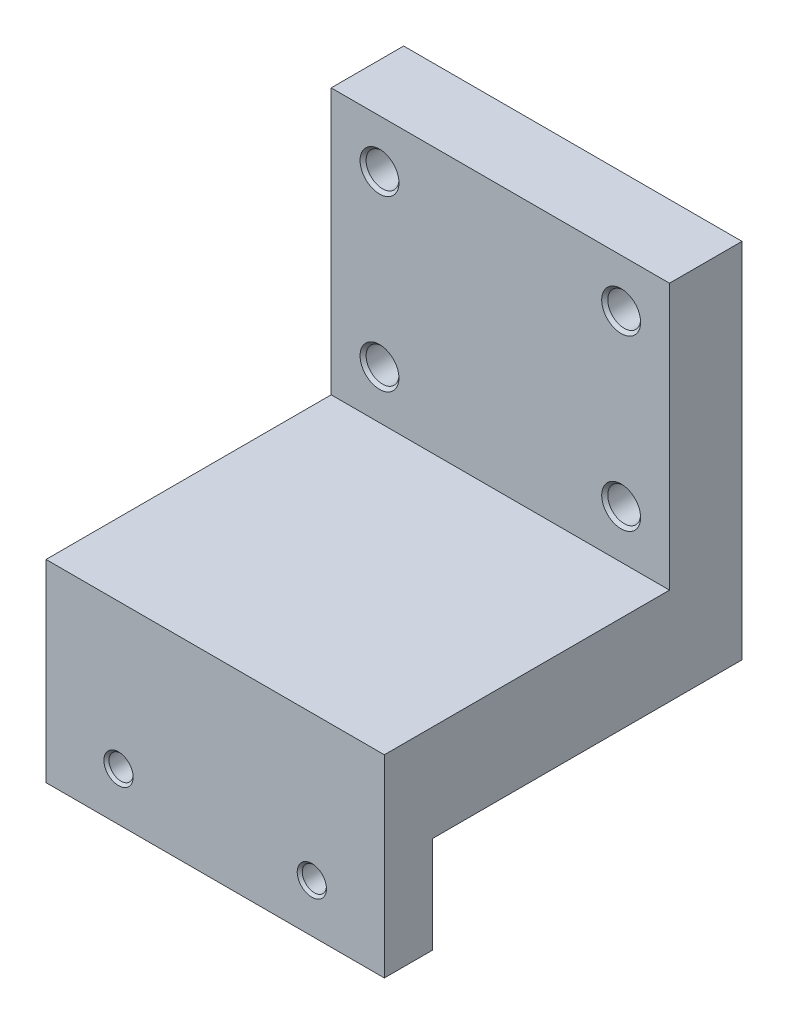
SolidWorks part; units mm, degrees
ref_plane "前视基准面" through (0, 0, 0) normal (0, 0, 1) x (1, 0, 0)
ref_plane "上视基准面" through (0, 0, 0) normal (0, 1, 0) x (1, 0, 0)
ref_plane "右视基准面" through (0, 0, 0) normal (1, 0, 0) x (0, 0, -1)
sketch "草图1" plane through (0, 0, 0) normal (0, 0, 1) x (1, 0, 0)
  line L0 (0, 0) -> (0, 45) construction
  line L1 (75, 35) -> (-75, 35) construction
  line L2 (-35, 55) -> (35, 55)
  line L3 (-35, 55) -> (-35, 35)
  line L4 (-35, 35) -> (35, 35)
  line L5 (35, 55) -> (35, 35)
  line L6 (-35, 55) -> (35, 35) construction
  line L7 (-35, 35) -> (35, 55) construction
  dimension "D1" = 20
  dimension "D2" = 70
extrude "凸台-拉伸1" add sketch "草图1" against normal blind 64 and the other way blind 10
sketch "草图2" plane through (0, 35, 0) normal (0, -1, 0) x (1, 0, 0)
  line L0 (35, 10) -> (35, -64) construction
  line L1 (-35, 10) -> (35, 10)
  line L2 (-35, 10) -> (-35, 0)
  line L3 (-35, 0) -> (35, 0)
  line L4 (35, 10) -> (35, 0)
  line L5 (-75, 0) -> (75, 0) construction
extrude "凸台-拉伸2" add sketch "草图2" along normal blind 20
sketch "草图3" plane through (0, 55, 0) normal (0, 1, 0) x (1, 0, 0)
  line L0 (-35, -10) -> (-35, 64) construction
  line L1 (35, 64) -> (-35, 64)
  line L2 (35, 64) -> (35, 49)
  line L3 (35, 49) -> (-35, 49)
  line L4 (-35, 64) -> (-35, 49)
  dimension "D1" = 15
extrude "凸台-拉伸3" add sketch "草图3" along normal blind 55
sketch "草图4" plane through (0, 0, -49) normal (0, 0, 1) x (1, 0, 0)
  line L8 (-25, 65) -> (25, 65)
  line L9 (25, 65) -> (25, 100)
  line L10 (25, 100) -> (-25, 100)
  line L11 (-25, 100) -> (-25, 65)
  line L12 (-25, 65) -> (25, 65)
  line L13 (25, 65) -> (25, 100)
  line L14 (25, 100) -> (-25, 100)
  line L15 (-25, 100) -> (-25, 65)
  dimension "D1" = 10
hole_wizard "M8 螺纹孔1" positions "草图7" profile "草图6" tap size "M8" standard "GB"
sketch "草图7" plane through (0, 0, -49) normal (0, 0, 1) x (1, 0, 0)
  point P0 (25, 100)
  point P3 (25, 65)
  point P6 (-25, 65)
  point P9 (-25, 100)
sketch "草图6" plane through (25, 100, -49) normal (1, 0, 0) x (0, -1, 0)
  line L0 (0, 0) -> (0, 19.75)
  line L1 (0, 19.75) -> (3.4, 17.7071)
  line L2 (3.4, 17.7071) -> (3.4, 0.625)
  line L3 (3.4, 0.625) -> (4.025, 0)
  line L5 (4.025, 0) -> (0, 0)
  line L6 (-3.4, 0.625) -> (-4.025, 0) construction
  line L10 (0, 19.75) -> (-3.4, 17.7071) construction
  line L11 (0, -6.35) -> (0, 107.95) construction
  dimension "螺纹孔钻头直径" = 6.8
  dimension "螺纹孔钻头深度" = 19.75
  dimension "近端锥形沉头孔直径" = 8.05
  dimension "近端锥形沉头孔角度" = 90
  dimension "导头角度" = 118
cosmetic thread "孔螺蚊线1" parameters "D1"=16, "D2"=8
cosmetic thread "孔螺蚊线2" parameters "D1"=16, "D2"=8
cosmetic thread "孔螺蚊线3" parameters "D1"=16, "D2"=8
cosmetic thread "孔螺蚊线4" parameters "D1"=16, "D2"=8
sketch "草图8" plane through (0, 0, 10) normal (0, 0, 1) x (1, 0, 0)
  line L0 (0, 0) -> (0, 25) construction
  line L1 (20, 25) -> (-20, 25)
  dimension "D1" = 20
  dimension "D2" = 25
hole_wizard "M6 螺纹孔1" positions "草图9" profile "草图10" tap size "M6" standard "GB"
sketch "草图9" plane through (0, 0, 10) normal (0, 0, 1) x (1, 0, 0)
  point P0 (20, 25)
  point P3 (-20, 25)
sketch "草图10" plane through (20, 25, 10) normal (1, 0, 0) x (0, -1, 0)
  line L0 (0, 0) -> (0, 15)
  line L1 (0, 15) -> (2.5, 13.4978)
  line L2 (2.5, 13.4978) -> (2.5, 0.525)
  line L3 (2.5, 0.525) -> (3.025, 0)
  line L5 (3.025, 0) -> (0, 0)
  line L6 (-2.5, 0.525) -> (-3.025, 0) construction
  line L10 (0, 15) -> (-2.5, 13.4978) construction
  line L11 (0, -6.35) -> (0, 107.95) construction
  dimension "螺纹孔钻头直径" = 5
  dimension "螺纹孔钻头深度" = 15
  dimension "近端锥形沉头孔直径" = 6.05
  dimension "近端锥形沉头孔角度" = 90
  dimension "导头角度" = 118
cosmetic thread "孔螺蚊线5" parameters "D1"=12, "D2"=6
cosmetic thread "孔螺蚊线6" parameters "D1"=12, "D2"=6
